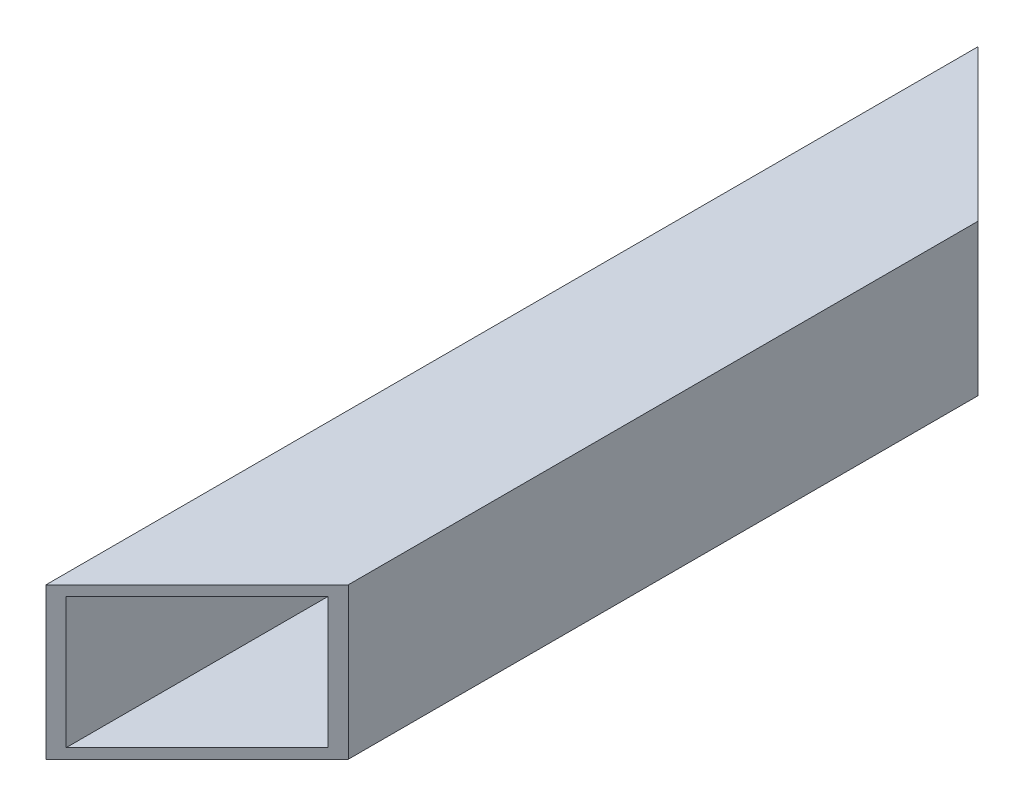
from build123d import *

# Parameters (mm, degrees)
SKETCH_1_W          = 30
SKETCH_1_H          = 30
SKETCH_1_W_2        = 26
SKETCH_1_H_2        = 26
EXTRUDE_1_DEPTH     = 92.5
CUT_EXTRUDE_1_DEPTH = 87


with BuildPart() as part:
    # 草图1 → 凸台-拉伸1 (new, symmetric)
    with BuildSketch(Plane.XY):
        Rectangle(SKETCH_1_W, SKETCH_1_H)
        Rectangle(SKETCH_1_W_2, SKETCH_1_H_2, mode=Mode.SUBTRACT)
    extrude(amount=EXTRUDE_1_DEPTH, both=True)

    # 草图2 → 切除-拉伸1 (cut)
    with BuildSketch(Plane(origin=(0, 15, 0), x_dir=(1, 0, 0), z_dir=(0, 1, 0))):
        Polygon((15, -62.5), (-15, -92.5), (15, -92.5), align=None)
        Polygon((15, 92.5), (-15, 92.5), (15, 62.5), align=None)
    extrude(amount=-CUT_EXTRUDE_1_DEPTH, mode=Mode.SUBTRACT)


solid = part.part
